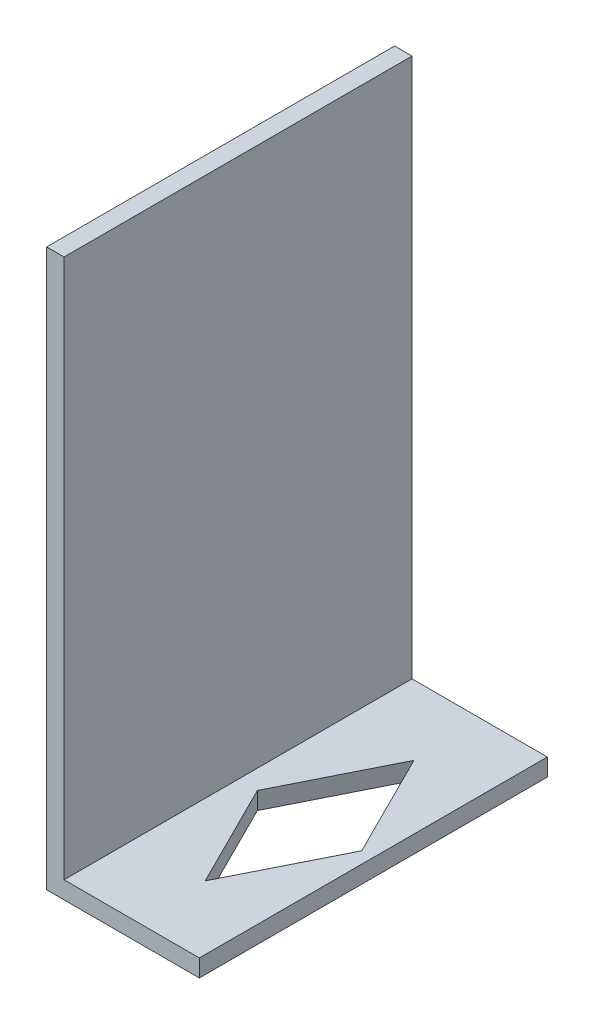
SolidWorks part; units mm, degrees
ref_plane "Front Plane" through (0, 0, 0) normal (0, 0, 1) x (1, 0, 0)
ref_plane "Top Plane" through (0, 0, 0) normal (0, 1, 0) x (1, 0, 0)
ref_plane "Right Plane" through (0, 0, 0) normal (1, 0, 0) x (0, 0, -1)
ref_plane "Plane4" through (0, 0, -180) normal (0, 0, 1) x (1, 0, 0)
sketch "Sketch2" plane through (0, 0, -180) normal (0, 0, 1) x (1, 0, 0)
  line L0 (-191.0157, 220) -> (-191.0157, -100)
  line L1 (-227.7505, 220) -> (0, 220) construction
  line L2 (-177.9115, -100) -> (-213.5052, -100) construction
  line L3 (-191.0157, -100) -> (-103.2543, -100)
  line L4 (-89.9115, -100) -> (-177.9115, -100) construction
  arc A0 (-229.3648, -67.8149) -> (-272.9623, 198.81) centre (-376.2555, 45.043) ccw construction
extrude "Extrude-Thin1" add sketch "Sketch2" along normal mid plane 200 thin thin type one direction reverse wall 10
sketch "Sketch3" plane through (0, -100, 0) normal (0, -1, 0) x (1, 0, 0)
  line L0 (-139.9115, -240) -> (-169.9115, -180) construction
  line L1 (-109.9115, -180) -> (-139.9115, -240) construction
  line L2 (-169.9115, -180) -> (-139.9115, -120) construction
  line L3 (-139.9115, -120) -> (-109.9115, -180) construction
  line L4 (-139.9115, -240) -> (-169.9115, -180)
  line L5 (-109.9115, -180) -> (-139.9115, -240)
  line L6 (-169.9115, -180) -> (-139.9115, -120)
  line L7 (-139.9115, -120) -> (-109.9115, -180)
extrude "Cut-Extrude1" cut sketch "Sketch3" against normal blind 79
